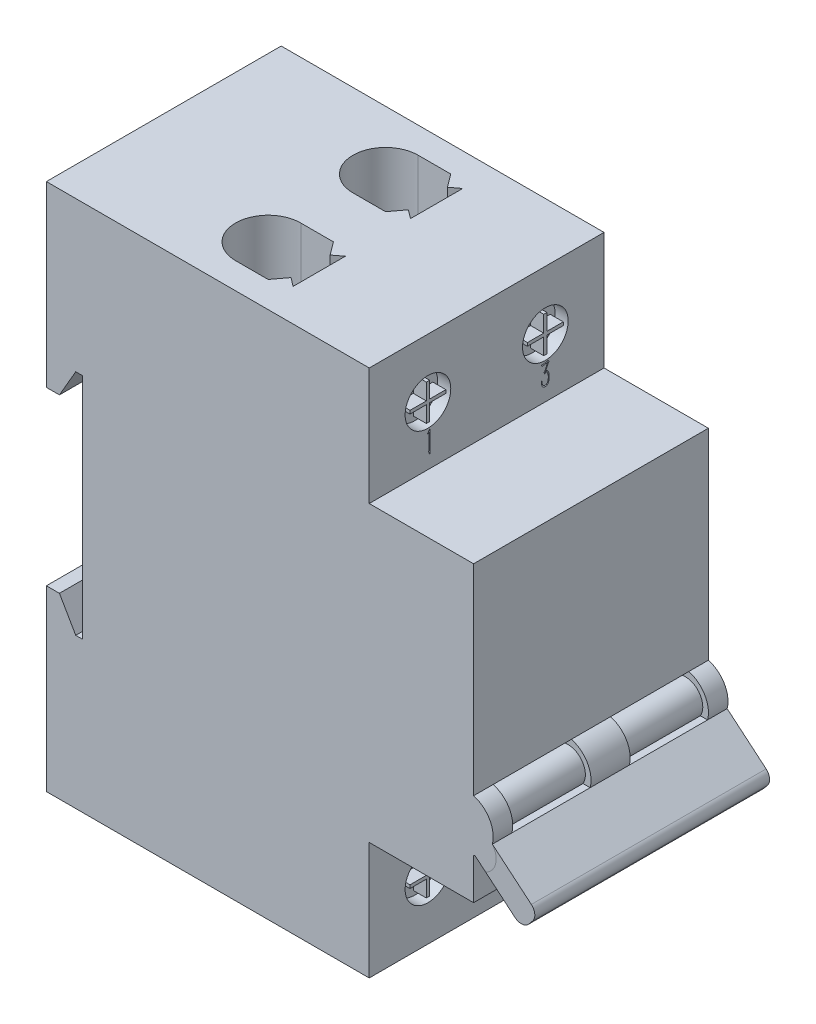
from build123d import *

# Parameters (mm, degrees)
EXTRUDE_1_DEPTH        = 18
SKETCH_2_R             = 3.5
CUT_EXTRUDE_1_DEPTH    = 2
CUT_EXTRUDE_5_DEPTH    = 15
SKETCH_12_R            = 4.114641301
EXTRUDE_4_DEPTH        = 18
EXTRUDE_5_DEPTH        = 18
FILLET_1_R             = 1.5
SKETCH_15_W            = 12
SKETCH_15_H            = 4.990244444
CUT_EXTRUDE_9_DEPTH    = 5
EXTRUDE_6_REACH        = 88.448
SKETCH_16_R            = 2.68605677
PATTERN_LINEAR_2_COUNT = 2
PATTERN_LINEAR_2_PITCH = 18
CUT_EXTRUDE_10_DEPTH   = 1


with BuildPart() as part:
    # 草图1 → 凸台-拉伸1 (new body)
    with BuildSketch(Plane.XY):
        Polygon((0, 13.169872981), (2, 13.169872981), (4.5, 17.5), (5.5, 17.5), (5.5, -17.5), (4.5, -17.5), (2, -13.169872981), (0, -13.169872981), (0, -40.5), (49.5, -40.5), (49.5, -22.5), (65.5, -22.5), (65.5, 22.5), (49.5, 22.5), (49.5, 40.5), (0, 40.5), align=None)
    extrude(amount=-EXTRUDE_1_DEPTH)

    # 草图2 → 切除-拉伸1 (cut)
    with BuildSketch(Plane(origin=(49.5, 0, 0), x_dir=(0, 0, -1), z_dir=(1, 0, 0))):
        with Locations((9, 31.5)):
            Circle(SKETCH_2_R)
        Polygon((8.75, 34.25), (9.25, 34.25), (9.25, 31.75), (11.75, 31.75), (11.75, 31.25), (9.25, 31.25), (9.25, 28.75), (8.75, 28.75), (8.75, 31.25), (6.25, 31.25), (6.25, 31.75), (8.75, 31.75), align=None, mode=Mode.SUBTRACT)
    cut_extrude_1 = extrude(amount=-CUT_EXTRUDE_1_DEPTH, mode=Mode.SUBTRACT)

    # 草图11 → 切除-拉伸5 (cut)
    with BuildSketch(Plane(origin=(0, 40.5, 0), x_dir=(1, 0, 0), z_dir=(0, 1, 0))):
        with BuildLine():
            Line((32.833333333, 5), (32.833333333, 13))
            Line((32.833333333, 13), (31.5, 12))
            Line((31.5, 12), (30, 14))
            Line((30, 14), (25, 14))
            ThreePointArc((25, 14), (21.464466094, 12.535533906), (20, 9))
            ThreePointArc((20, 9), (21.464466094, 5.464466094), (25, 4))
            Line((25, 4), (30, 4))
            Line((30, 4), (31.5, 6))
            Line((31.5, 6), (32.833333333, 5))
        make_face()
    cut_extrude_5 = extrude(amount=-CUT_EXTRUDE_5_DEPTH, mode=Mode.SUBTRACT)

    # 镜向1: 切除-拉伸1, 切除-拉伸5 across plane
    add(cut_extrude_1.mirror(Plane.ZX), mode=Mode.SUBTRACT)
    add(cut_extrude_5.mirror(Plane.ZX), mode=Mode.SUBTRACT)

    # 草图12 → 凸台-拉伸4 (add, through all)
    with BuildSketch(Plane.XY):
        with Locations((64.39025967, -12.26560275)):
            Circle(SKETCH_12_R)
    extrude(amount=-EXTRUDE_4_DEPTH)

    # 草图13 → 凸台-拉伸5 (add, through all)
    with BuildSketch(Plane.XY):
        Polygon((65.5, -10.881779635), (75.5, -19.272775947), (72.999147741, -22.253175611), (65.5, -15.960643508), align=None)
    extrude(amount=-EXTRUDE_5_DEPTH)

    # 圆角1
    fillet_1_edges = [part.edges().sort_by_distance(p)[0] for p in [
        (75.5, -19.272775947, -9),
        (72.999147741, -22.253175611, -9),
    ]]
    fillet(fillet_1_edges, radius=FILLET_1_R)

    # 草图15 → 切除-拉伸9 (cut, symmetric)
    with BuildSketch(Plane(origin=(65.5, 0, 0), x_dir=(0, 0, -1), z_dir=(1, 0, 0))):
        with Locations((9, -10.798560231)):
            Rectangle(SKETCH_15_W, SKETCH_15_H)
    extrude(amount=CUT_EXTRUDE_9_DEPTH, both=True, mode=Mode.SUBTRACT)

    # 草图16 → 凸台-拉伸6 (add, up to next)
    with BuildSketch(Plane.XY.offset(-15), mode=Mode.PRIVATE) as extrude_6_sk1:
        with Locations((64.953909061, -11.94282373)):
            Circle(SKETCH_16_R)
    extrude_6_tool1 = extrude(extrude_6_sk1.sketch, amount=EXTRUDE_6_REACH, mode=Mode.PRIVATE) - part.part
    add(extrude_6_tool1.solids().sort_by_distance((64.953909, -11.942824, -15))[0])


with BuildPart() as pattern_linear_2_1:
    # 阵列(线性)2: pattern copy
    add(part.part.moved(Location(Vector(0, 0, -1) * (1 * PATTERN_LINEAR_2_PITCH))))


with BuildPart() as part_1:
    add(part.part)

    # Combine 1: union 阵列(线性)2_1
    add(pattern_linear_2_1.part)

    # 草图19 → 切除-拉伸10 (cut)
    # profile 1 of 4: a face of its own
    with BuildSketch(Plane(origin=(49.5, 0, 0), x_dir=(0, 0, -1), z_dir=(1, 0, 0))):
        with BuildLine():
            Line((9.268616193, 27.777022397), (9.323804772, 27.777022397))
            Line((9.323804772, 27.777022397), (9.31858423, 25.103359495))
            add(Edge.make_bspline(
                [(9.31858423, 25.103359495), (9.317989513, 25.079247206), (9.316849208, 25.033014576), (9.316756663, 24.966867672), (9.314581251, 24.906977786), (9.31440798, 24.853259172), (9.312790378, 24.805782007), (9.310919778, 24.764536358), (9.310742036, 24.729444909), (9.307433278, 24.674522263), (9.303490456, 24.59900772), (9.293712461, 24.521229024), (9.285928441, 24.465808449), (9.278015344, 24.440580035), (9.267990261, 24.420618486), (9.257985248, 24.422946371), (9.253700361, 24.423943344)],
                knots=[0, 0, 0, 0, 1.45038606, 2.780953852, 3.977268029, 5.053718292, 6.010937745, 6.833690271, 7.536464333, 8.120251454, 10.142880859, 12.069479857, 12.873132744, 13.440417135, 13.76034519, 14, 14, 14, 14], degree=3))
            add(Edge.make_bspline(
                [(9.253700361, 24.423943344), (9.252709832, 24.424693106), (9.248470125, 24.427902274), (9.238359598, 24.434694901), (9.226346206, 24.452902941), (9.221087494, 24.469237998), (9.217902364, 24.479131922)],
                knots=[0, 0, 0, 0, 0.221265066, 0.947068446, 2.150880552, 4, 4, 4, 4], degree=3))
            Line((9.217902364, 24.479131922), (9.193291241, 24.544761583))
            Line((9.193291241, 24.544761583), (9.13735687, 24.725988943))
            add(Edge.make_bspline(
                [(9.13735687, 24.725988943), (9.130623579, 24.743040571), (9.118894532, 24.772743625), (9.107062513, 24.811822119), (9.098086344, 24.836775388), (9.09570055, 24.857001098), (9.107192928, 24.875972867), (9.11565667, 24.905183607), (9.128680107, 24.942469195), (9.140978693, 24.986476292), (9.151841244, 25.034025265), (9.161626509, 25.085400436), (9.167172099, 25.143283169), (9.169892428, 25.198549028), (9.171980118, 25.251758462), (9.172359418, 25.302984326), (9.173405582, 25.363637315), (9.173242151, 25.407393199), (9.173154868, 25.43076201)],
                knots=[0, 0, 0, 0, 1.220359697, 2.125803599, 2.712350858, 2.994193817, 3.439826662, 4.12562012, 5.031064022, 6.063176816, 7.167225426, 8.277459231, 9.542238136, 11.034069985, 11.961482632, 13.08703073, 14.444263491, 16, 16, 16, 16], degree=3))
            Line((9.173154868, 25.43076201), (9.177629617, 27.404126595))
            Line((9.177629617, 27.404126595), (8.915856764, 27.177405947))
            Line((8.915856764, 27.177405947), (8.895720391, 27.263171982))
            add(Edge.make_bspline(
                [(8.895720391, 27.263171982), (8.916998829, 27.285159101), (8.956886141, 27.326374863), (9.010193269, 27.385718152), (9.054036517, 27.437218727), (9.099702186, 27.497425312), (9.150830111, 27.572352034), (9.188586471, 27.633910013), (9.208207073, 27.665899448)],
                knots=[0, 0, 0, 0, 1.077185482, 2.019228619, 2.808185376, 3.45765616, 4.678836699, 6, 6, 6, 6], degree=3))
            Line((9.208207073, 27.665899448), (9.268616193, 27.777022397))
        make_face()
    # profile 2 of 4: a face of its own
    with BuildSketch(Plane(origin=(49.5, 0, 0), x_dir=(0, 0, -1), z_dir=(1, 0, 0))):
        with BuildLine():
            add(Edge.make_bspline(
                [(26.894587034, 26.553178374), (26.905758668, 26.576305419), (26.92727936, 26.620856647), (26.95866931, 26.685209589), (26.987953271, 26.744293665), (27.012999895, 26.799120123), (27.036354733, 26.848480227), (27.057155241, 26.892902394), (27.075128281, 26.932401147), (27.094050096, 26.976253222), (27.113674908, 27.02200111), (27.132673375, 27.066809999), (27.146489283, 27.098818021), (27.153632136, 27.115750937), (27.156359887, 27.122217369)],
                knots=[0, 0, 0, 0, 1.475873638, 2.843077615, 4.114458223, 5.26483622, 6.306479236, 7.252326145, 8.083448402, 8.799989154, 9.996708352, 10.943956596, 11.596712522, 12, 12, 12, 12], degree=3))
            Line((27.156359887, 27.122217369), (27.317450874, 27.55030175))
            add(Edge.make_bspline(
                [(27.317450874, 27.55030175), (27.282414717, 27.546873059), (27.20596755, 27.539391824), (27.108407493, 27.533451709), (27.027289802, 27.529125888), (26.971629196, 27.524461766), (26.922889389, 27.520102343), (26.892842398, 27.516785719), (26.87892541, 27.515249544)],
                knots=[0, 0, 0, 0, 1.440114021, 3.142257811, 3.998086789, 4.76330671, 5.427195687, 6, 6, 6, 6], degree=3))
            Line((26.87892541, 27.515249544), (26.728275506, 27.48989263))
            add(Edge.make_bspline(
                [(26.728275506, 27.48989263), (26.721544061, 27.488477454), (26.70317884, 27.484616469), (26.669215876, 27.474073313), (26.620302936, 27.461107664), (26.58307352, 27.450445131), (26.561963978, 27.444399342)],
                knots=[0, 0, 0, 0, 0.478461291, 1.305373098, 2.472113022, 4, 4, 4, 4], degree=3))
            Line((26.561963978, 27.444399342), (26.511995941, 27.424262968))
            Line((26.511995941, 27.424262968), (26.38595716, 27.61071087))
            add(Edge.make_bspline(
                [(26.38595716, 27.61071087), (26.380634962, 27.618010698), (26.371549402, 27.630472284), (26.364006769, 27.647807605), (26.358407972, 27.65985087), (26.363426008, 27.671978454), (26.383268796, 27.670159902), (26.398250403, 27.659523203), (26.417386103, 27.649289333), (26.439402155, 27.647850003), (26.466093406, 27.646283592), (26.485655754, 27.64932396), (26.496334317, 27.650983616)],
                knots=[0, 0, 0, 0, 1.323589942, 2.259509366, 2.829398404, 3.190947808, 3.965341466, 5.19662492, 6.050472624, 7.088782, 8.410843841, 10, 10, 10, 10], degree=3))
            Line((26.496334317, 27.650983616), (26.657425304, 27.656204158))
            Line((26.657425304, 27.656204158), (27.292093959, 27.73152911))
            Line((27.292093959, 27.73152911), (27.342061997, 27.777022397))
            Line((27.342061997, 27.777022397), (27.382334743, 27.817295144))
            add(Edge.make_bspline(
                [(27.382334743, 27.817295144), (27.383583719, 27.815808411), (27.388703828, 27.809713632), (27.399726504, 27.795210802), (27.419326367, 27.771910062), (27.434144734, 27.752492469), (27.442743863, 27.7412244)],
                knots=[0, 0, 0, 0, 0.23984028, 0.983211964, 2.249351781, 4, 4, 4, 4], degree=3))
            Line((27.442743863, 27.7412244), (27.53895098, 27.62040616))
            add(Edge.make_bspline(
                [(27.53895098, 27.62040616), (27.54541144, 27.612018118), (27.556147701, 27.598078521), (27.564112726, 27.575785092), (27.555951012, 27.56068078), (27.544549588, 27.547733644), (27.52606782, 27.532183142), (27.511424617, 27.521362113), (27.503152983, 27.515249544)],
                knots=[0, 0, 0, 0, 1.419029252, 2.358201718, 2.827787952, 3.596253847, 4.642174893, 6, 6, 6, 6], degree=3))
            Line((27.503152983, 27.515249544), (27.447964405, 27.469756256))
            add(Edge.make_bspline(
                [(27.447964405, 27.469756256), (27.43183587, 27.429222959), (27.401234241, 27.352316717), (27.357143356, 27.242865851), (27.316798395, 27.145548297), (27.281372724, 27.059514144), (27.248833746, 26.985741252), (27.221970898, 26.923143149), (27.197785591, 26.872921774), (27.182992591, 26.843523203), (27.176496261, 26.830612851)],
                knots=[0, 0, 0, 0, 1.507300768, 2.859891598, 4.076963614, 5.147345159, 6.074452096, 6.862861548, 7.500626815, 8, 8, 8, 8], degree=3))
            Line((27.176496261, 26.830612851), (27.025100565, 26.543483084))
            add(Edge.make_bspline(
                [(27.025100565, 26.543483084), (27.042996023, 26.54491193), (27.077268983, 26.547648422), (27.129573753, 26.552872254), (27.186562807, 26.54568692), (27.236547135, 26.525696313), (27.279075075, 26.501029434), (27.313152721, 26.476392071), (27.345708772, 26.444370394), (27.378905936, 26.406726573), (27.412180649, 26.361796719), (27.442768582, 26.307377441), (27.474610228, 26.245235491), (27.514431877, 26.150532156), (27.557460863, 26.023817162), (27.583604576, 25.86466242), (27.596521571, 25.705205737), (27.598417879, 25.599087053), (27.5993601, 25.546359708)],
                knots=[0, 0, 0, 0, 0.660541429, 1.265053373, 1.928435853, 2.750244091, 3.225390118, 3.735570922, 4.291687282, 4.900607759, 5.580848831, 6.342918567, 7.193367346, 8.147740655, 10.119512469, 12.097611575, 14.061014616, 16, 16, 16, 16], degree=3))
            add(Edge.make_bspline(
                [(27.5993601, 25.546359708), (27.597369738, 25.505079829), (27.593588689, 25.426661312), (27.584450789, 25.315849931), (27.570814377, 25.218634004), (27.550955275, 25.109031476), (27.515932295, 24.987942252), (27.472665848, 24.876226259), (27.431585008, 24.795741244), (27.396962993, 24.742372127), (27.359042011, 24.69462663), (27.318290969, 24.652844146), (27.275901478, 24.618507711), (27.234760539, 24.588977252), (27.193130085, 24.568106084), (27.139235736, 24.550670286), (27.073375552, 24.538651683), (27.020920749, 24.536243809), (26.995268901, 24.535066293)],
                knots=[0, 0, 0, 0, 1.512752116, 2.8737433, 4.067977017, 5.104892351, 6.948544146, 8.672095895, 9.482011449, 10.251829035, 10.996496654, 11.710742831, 12.38300564, 12.991319199, 13.561044299, 14.079002633, 15.060579187, 16, 16, 16, 16], degree=3))
            add(Edge.make_bspline(
                [(26.995268901, 24.535066293), (26.973388966, 24.534693339), (26.93129448, 24.53397582), (26.870237534, 24.538946321), (26.81462808, 24.55032289), (26.762475647, 24.565798969), (26.713633203, 24.590272598), (26.666979223, 24.625233083), (26.620013623, 24.668282899), (26.574983014, 24.721112889), (26.533770386, 24.781638563), (26.497735149, 24.848588226), (26.46779483, 24.921014069), (26.438030374, 25.024086001), (26.412802475, 25.155884677), (26.408308057, 25.262588435), (26.406093533, 25.315164311)],
                knots=[0, 0, 0, 0, 0.828828519, 1.594571005, 2.314948186, 2.97625877, 3.650192192, 4.371738268, 5.178272596, 6.059897072, 6.995131469, 7.947518938, 8.935744196, 9.957858231, 12.008325587, 14, 14, 14, 14], degree=3))
            Line((26.406093533, 25.315164311), (26.400872992, 25.511307503))
            Line((26.400872992, 25.511307503), (26.456061571, 25.511307503))
            add(Edge.make_bspline(
                [(26.456061571, 25.511307503), (26.460281768, 25.482221028), (26.468363821, 25.426517849), (26.480120095, 25.346152318), (26.492296408, 25.272893692), (26.50601877, 25.186199105), (26.528872927, 25.088850434), (26.567375212, 24.984077852), (26.619589704, 24.89555163), (26.680895946, 24.822599949), (26.752597249, 24.769647856), (26.829354682, 24.736246775), (26.90758436, 24.720476219), (26.959416586, 24.720672281), (26.984827818, 24.720768402)],
                knots=[0, 0, 0, 0, 0.994021113, 1.903638599, 2.746793397, 3.505624798, 4.871908371, 6.122639036, 7.264652637, 8.331625701, 9.323760524, 10.250011688, 11.142051883, 12, 12, 12, 12], degree=3))
            add(Edge.make_bspline(
                [(26.984827818, 24.720768402), (27.005270774, 24.722531252), (27.045310018, 24.725983941), (27.103371268, 24.739128694), (27.157066245, 24.761557691), (27.207260378, 24.790239493), (27.252440104, 24.827641551), (27.293102101, 24.871713388), (27.327537611, 24.924069674), (27.366130118, 25.004224122), (27.403636112, 25.114727617), (27.431856393, 25.255086396), (27.450219792, 25.398256076), (27.458846817, 25.540709206), (27.460022294, 25.681050273), (27.448482407, 25.772899132), (27.442743863, 25.818573644)],
                knots=[0, 0, 0, 0, 0.647840119, 1.268849254, 1.871153999, 2.479976942, 3.088343857, 3.716462885, 4.367721208, 5.059616847, 6.52246665, 8.039623249, 9.575767262, 11.078710543, 12.547304005, 14, 14, 14, 14], degree=3))
            add(Edge.make_bspline(
                [(27.442743863, 25.818573644), (27.434719682, 25.867804036), (27.418857721, 25.965121191), (27.382165945, 26.081930294), (27.346034778, 26.169154367), (27.313799504, 26.227674778), (27.277262229, 26.279947351), (27.235874793, 26.32378913), (27.193919543, 26.35976614), (27.15180766, 26.383772702), (27.110219955, 26.396125961), (27.083571503, 26.393410031), (27.070593853, 26.392087388)],
                knots=[0, 0, 0, 0, 2.019199264, 3.991492233, 4.943861116, 5.841091039, 6.693606335, 7.520378909, 8.278781735, 8.923571305, 9.475785111, 10, 10, 10, 10], degree=3))
            Line((27.070593853, 26.392087388), (26.990048359, 26.382392097))
            Line((26.990048359, 26.382392097), (26.954996154, 26.316762436))
            add(Edge.make_bspline(
                [(26.954996154, 26.316762436), (26.950317629, 26.308583345), (26.94216181, 26.294325183), (26.931016972, 26.275479105), (26.922115728, 26.264440522), (26.915359483, 26.254924454), (26.905592767, 26.258125672), (26.899310799, 26.269064642), (26.889268494, 26.285168339), (26.882736067, 26.298999064), (26.87892541, 26.307067145)],
                knots=[0, 0, 0, 0, 1.659028505, 2.892093886, 3.763458346, 4.288089223, 4.647361994, 5.327919393, 6.441255868, 8, 8, 8, 8], degree=3))
            Line((26.87892541, 26.307067145), (26.798379917, 26.46293759))
            add(Edge.make_bspline(
                [(26.798379917, 26.46293759), (26.792557932, 26.471896017), (26.782408552, 26.48751311), (26.786808583, 26.505315301), (26.788684626, 26.512905628)],
                knots=[0, 0, 0, 0, 1.147259222, 2, 2, 2, 2], degree=3))
            Line((26.788684626, 26.512905628), (26.828957373, 26.528567251))
            Line((26.828957373, 26.528567251), (26.894587034, 26.553178374))
        make_face()
    # profile 3 of 4: a face of its own
    with BuildSketch(Plane(origin=(49.5, 0, 0), x_dir=(0, 0, -1), z_dir=(1, 0, 0))):
        with BuildLine():
            Line((8.730154654, -24.847385713), (8.654083911, -24.847385713))
            add(Edge.make_bspline(
                [(8.654083911, -24.847385713), (8.652516507, -24.823276458), (8.649528375, -24.777314072), (8.646445032, -24.711674798), (8.64514292, -24.652738754), (8.643838503, -24.580888811), (8.645850242, -24.490276951), (8.65125193, -24.417292602), (8.654083911, -24.379028585)],
                knots=[0, 0, 0, 0, 0.927540379, 1.768282303, 2.522502339, 3.190652681, 4.527123766, 6, 6, 6, 6], degree=3))
            add(Edge.make_bspline(
                [(8.654083911, -24.379028585), (8.656043818, -24.350662308), (8.659834054, -24.295805178), (8.669837058, -24.216742672), (8.681413565, -24.143478296), (8.69646412, -24.074567742), (8.7167999, -24.007131882), (8.745750083, -23.939303027), (8.781856415, -23.868757962), (8.824515086, -23.797966017), (8.871321724, -23.731168134), (8.923860232, -23.676810886), (8.978846052, -23.635379689), (9.03734966, -23.610721813), (9.093521598, -23.595388131), (9.144745804, -23.583326557), (9.190777383, -23.574897147), (9.219860114, -23.573997547), (9.233563987, -23.573573652)],
                knots=[0, 0, 0, 0, 1.238521709, 2.395159043, 3.470603583, 4.46912877, 5.466066804, 6.534123646, 7.677244524, 8.916145015, 10.13365226, 11.221244199, 12.198275335, 13.109907183, 13.966820176, 14.733954848, 15.403435577, 16, 16, 16, 16], degree=3))
            add(Edge.make_bspline(
                [(9.233563987, -23.573573652), (9.251028183, -23.574861334), (9.285536892, -23.577405754), (9.336298249, -23.589194749), (9.3853233, -23.606192719), (9.448027995, -23.63647274), (9.521351042, -23.683947637), (9.583729421, -23.746290041), (9.626893488, -23.803356357), (9.65729834, -23.851924205), (9.684241838, -23.90615696), (9.718077941, -23.984958998), (9.75347521, -24.089530022), (9.779001912, -24.221603947), (9.795369003, -24.35875684), (9.802857469, -24.498968402), (9.804249869, -24.637798018), (9.796098136, -24.728340443), (9.792161899, -24.772060761)],
                knots=[0, 0, 0, 0, 0.570779476, 1.127842599, 1.694919432, 2.261066821, 3.397481896, 4.527710891, 5.118384485, 5.730727279, 6.394748858, 7.092559246, 8.529363642, 9.986910621, 11.474321506, 13.03467297, 14.568129345, 16, 16, 16, 16], degree=3))
            add(Edge.make_bspline(
                [(9.792161899, -24.772060761), (9.784182525, -24.817033009), (9.768104722, -24.907648497), (9.733475036, -25.016748296), (9.701178927, -25.099692259), (9.674177686, -25.155273163), (9.645327126, -25.204477751), (9.603609389, -25.262667052), (9.539900956, -25.328718412), (9.480864698, -25.373013219), (9.449843553, -25.396288334)],
                knots=[0, 0, 0, 0, 1.490916612, 3.004077927, 3.729534125, 4.397912905, 5.020560084, 5.590839424, 6.734084393, 8, 8, 8, 8], degree=3))
            Line((9.449843553, -25.396288334), (9.202986532, -25.552158779))
            add(Edge.make_bspline(
                [(9.202986532, -25.552158779), (9.171529528, -25.573514544), (9.111881044, -25.614009149), (9.032233852, -25.680155183), (8.965383351, -25.749851267), (8.914854257, -25.826914516), (8.875609345, -25.906240314), (8.840761113, -25.985891172), (8.814452469, -26.073684748), (8.795740738, -26.152376603), (8.782979957, -26.218465922), (8.776587827, -26.264558022), (8.771395086, -26.305294785), (8.770736473, -26.330751604), (8.770427401, -26.34269788)],
                knots=[0, 0, 0, 0, 1.453572249, 2.75625039, 3.953730064, 5.132566341, 6.263730064, 7.337486329, 8.453238547, 9.76321854, 10.430854957, 11.026567013, 11.543191201, 12, 12, 12, 12], degree=3))
            Line((8.770427401, -26.34269788), (8.759986319, -26.553756904))
            Line((8.759986319, -26.553756904), (9.660902577, -26.52392524))
            add(Edge.make_bspline(
                [(9.660902577, -26.52392524), (9.672462855, -26.523278875), (9.692767296, -26.522143602), (9.71228111, -26.500870216), (9.71662466, -26.474895395), (9.724332018, -26.442947113), (9.730061911, -26.397152102), (9.734482123, -26.362325748), (9.736973321, -26.34269788)],
                knots=[0, 0, 0, 0, 0.925905201, 1.626257371, 2.181371879, 3.087088273, 4.358305093, 6, 6, 6, 6], degree=3))
            Line((9.736973321, -26.34269788), (9.757109694, -25.904172416))
            Line((9.757109694, -25.904172416), (9.827214105, -25.904172416))
            Line((9.827214105, -25.904172416), (9.852571019, -26.568672736))
            add(Edge.make_bspline(
                [(9.852571019, -26.568672736), (9.853418715, -26.581591346), (9.854901335, -26.604186009), (9.855623054, -26.634075483), (9.855643482, -26.654888005), (9.855328713, -26.671692005), (9.849916523, -26.68638406), (9.84488751, -26.703431679), (9.825269802, -26.713062781), (9.797070739, -26.716144309), (9.754214435, -26.720508585), (9.720578586, -26.720229453), (9.701175324, -26.720068432)],
                knots=[0, 0, 0, 0, 1.385018147, 2.4223982, 3.193529914, 3.619812046, 4.200562765, 4.878496499, 5.402948042, 6.404258339, 7.925751149, 10, 10, 10, 10], degree=3))
            Line((9.701175324, -26.720068432), (8.699577199, -26.745425346))
            add(Edge.make_bspline(
                [(8.699577199, -26.745425346), (8.687401759, -26.745460965), (8.663403069, -26.745531172), (8.638810076, -26.721667198), (8.628486444, -26.692453054), (8.623319507, -26.658091359), (8.61985857, -26.612504766), (8.618196149, -26.534098628), (8.621750352, -26.422538741), (8.629756092, -26.330484316), (8.633947537, -26.28228876)],
                knots=[0, 0, 0, 0, 0.556373901, 1.096654043, 1.476064089, 2.012759395, 2.73145082, 3.635924119, 5.715166189, 8, 8, 8, 8], degree=3))
            add(Edge.make_bspline(
                [(8.633947537, -26.28228876), (8.637667097, -26.254157079), (8.644832261, -26.199965695), (8.659400716, -26.121959966), (8.674933052, -26.049553187), (8.691789735, -25.982789164), (8.710398684, -25.922019627), (8.7307103, -25.867314144), (8.751766421, -25.81779166), (8.783393806, -25.761768771), (8.82358975, -25.700701936), (8.86931043, -25.634857188), (8.91333054, -25.579003158), (8.970866969, -25.517554724), (9.048760279, -25.450483145), (9.114195614, -25.401371673), (9.147797953, -25.37615196)],
                knots=[0, 0, 0, 0, 1.103491021, 2.125706759, 3.085324024, 3.98349739, 4.803138144, 5.555704107, 6.252741852, 6.89323317, 8.054555834, 9.09539633, 10.010480884, 10.817709087, 12.365830683, 14, 14, 14, 14], degree=3))
            Line((9.147797953, -25.37615196), (9.354382227, -25.244892638))
            add(Edge.make_bspline(
                [(9.354382227, -25.244892638), (9.370921509, -25.233896319), (9.402660187, -25.212794517), (9.446498042, -25.179198736), (9.483871457, -25.144340724), (9.516078649, -25.106724377), (9.545234203, -25.063196929), (9.569178512, -25.008940647), (9.59449199, -24.945031971), (9.624006101, -24.845602012), (9.654437281, -24.714363208), (9.666102897, -24.552212497), (9.65987102, -24.387958902), (9.640818996, -24.278938888), (9.631070913, -24.22315814)],
                knots=[0, 0, 0, 0, 0.635613896, 1.219735276, 1.765761318, 2.268061313, 2.802129131, 3.435697723, 4.161225462, 5.001884758, 6.75303811, 8.46119913, 10.189351173, 12, 12, 12, 12], degree=3))
            add(Edge.make_bspline(
                [(9.631070913, -24.22315814), (9.623725567, -24.194721139), (9.609399703, -24.139259545), (9.582284963, -24.059364957), (9.547186593, -23.986598886), (9.509619076, -23.918624202), (9.462554079, -23.859122868), (9.399862794, -23.816389074), (9.325801546, -23.787822518), (9.27162761, -23.782792113), (9.243259278, -23.780157927)],
                knots=[0, 0, 0, 0, 1.101106684, 2.147523679, 3.156537618, 4.125318695, 5.058520457, 5.968677808, 6.93629249, 8, 8, 8, 8], degree=3))
            add(Edge.make_bspline(
                [(9.243259278, -23.780157927), (9.228326882, -23.78000505), (9.198543172, -23.779700127), (9.15418165, -23.786427429), (9.111033958, -23.800532746), (9.054355541, -23.826097853), (8.988862492, -23.873718727), (8.91992613, -23.945569602), (8.863064593, -24.033301084), (8.819285565, -24.13496587), (8.786366995, -24.250789776), (8.759643561, -24.380596909), (8.742096183, -24.52603338), (8.737193746, -24.627827981), (8.734629404, -24.681074185)],
                knots=[0, 0, 0, 0, 0.469335518, 0.936122588, 1.403629858, 1.893624907, 2.887406355, 3.927357629, 5.011993806, 6.157121359, 7.396943717, 8.794309501, 10.323183677, 12, 12, 12, 12], degree=3))
            Line((8.734629404, -24.681074185), (8.730154654, -24.847385713))
        make_face()
    # profile 4 of 4: a face of its own
    with BuildSketch(Plane(origin=(49.5, 0, 0), x_dir=(0, 0, -1), z_dir=(1, 0, 0))):
        with BuildLine():
            Line((27.186191551, -25.808711091), (26.476197944, -25.848983838))
            Line((26.476197944, -25.848983838), (26.426229906, -25.92430879))
            add(Edge.make_bspline(
                [(26.426229906, -25.92430879), (26.422969209, -25.932202289), (26.418041285, -25.944131812), (26.399821496, -25.956434612), (26.386153034, -25.938787294), (26.379694111, -25.927278587), (26.375516077, -25.91983404)],
                knots=[0, 0, 0, 0, 1.282902353, 1.938863145, 2.666728425, 4, 4, 4, 4], degree=3))
            Line((26.375516077, -25.91983404), (26.280054752, -25.728165598))
            add(Edge.make_bspline(
                [(26.280054752, -25.728165598), (26.275970963, -25.716847246), (26.269236836, -25.698183401), (26.264334142, -25.673131982), (26.265728107, -25.655463636), (26.268963559, -25.646337108), (26.270359461, -25.642399563)],
                knots=[0, 0, 0, 0, 1.63130738, 2.690008936, 3.434818089, 4, 4, 4, 4], degree=3))
            Line((26.270359461, -25.642399563), (26.310632208, -25.632704272))
            Line((26.310632208, -25.632704272), (26.365820786, -25.602126817))
            Line((26.365820786, -25.602126817), (27.216769007, -23.548216738))
            Line((27.216769007, -23.548216738), (27.327146165, -23.548216738))
            Line((27.327146165, -23.548216738), (27.327146165, -25.62226319))
            add(Edge.make_bspline(
                [(27.327146165, -25.62226319), (27.337517711, -25.622341822), (27.355153283, -25.622475527), (27.371235704, -25.615458278), (27.377859994, -25.612567899)],
                knots=[0, 0, 0, 0, 1.176207474, 2, 2, 2, 2], degree=3))
            Line((27.377859994, -25.612567899), (27.453184946, -25.581990443))
            add(Edge.make_bspline(
                [(27.453184946, -25.581990443), (27.462922591, -25.578356102), (27.480279634, -25.571878005), (27.502629071, -25.562149087), (27.518450332, -25.554658262), (27.525822287, -25.549000794), (27.528509898, -25.546938238)],
                knots=[0, 0, 0, 0, 1.495147538, 2.665053038, 3.513315187, 4, 4, 4, 4], degree=3))
            Line((27.528509898, -25.546938238), (27.563562103, -25.517106574))
            Line((27.563562103, -25.517106574), (27.704516717, -25.662535937))
            add(Edge.make_bspline(
                [(27.704516717, -25.662535937), (27.711697463, -25.671177462), (27.723452054, -25.685323286), (27.728582435, -25.70926226), (27.723689862, -25.725451473), (27.714543829, -25.737110002), (27.698601358, -25.741996953), (27.686866477, -25.742677653), (27.679905594, -25.74308143)],
                knots=[0, 0, 0, 0, 1.690587597, 2.767423091, 3.557953073, 4.202677464, 4.933866242, 6, 6, 6, 6], degree=3))
            Line((27.679905594, -25.74308143), (27.327146165, -25.783354176))
            Line((27.327146165, -25.783354176), (27.327146165, -26.685016226))
            add(Edge.make_bspline(
                [(27.327146165, -26.685016226), (27.327128212, -26.687751147), (27.327067793, -26.696955205), (27.328226229, -26.716330922), (27.328695969, -26.747160979), (27.329300443, -26.7854712), (27.330335667, -26.823912608), (27.330001199, -26.855048118), (27.327983039, -26.874682486), (27.323236362, -26.887300824), (27.313944894, -26.889560225), (27.309175758, -26.887373218), (27.307009791, -26.88637996)],
                knots=[0, 0, 0, 0, 0.375701713, 1.264380521, 2.665139726, 4.612257271, 6.525225464, 7.960129458, 8.858599367, 9.286556546, 9.675980055, 10, 10, 10, 10], degree=3))
            add(Edge.make_bspline(
                [(27.307009791, -26.88637996), (27.302798935, -26.883877082), (27.290105158, -26.876332067), (27.278979998, -26.851983484), (27.265612394, -26.826711093), (27.259603022, -26.808412858), (27.257041754, -26.800613925)],
                knots=[0, 0, 0, 0, 0.572299195, 1.725216547, 3.030459198, 4, 4, 4, 4], degree=3))
            Line((27.257041754, -26.800613925), (27.211548466, -26.709627349))
            Line((27.211548466, -26.709627349), (27.186191551, -26.639522938))
            add(Edge.make_bspline(
                [(27.186191551, -26.639522938), (27.182335483, -26.631121959), (27.175357852, -26.615920221), (27.167714287, -26.594965646), (27.160889762, -26.579495575), (27.157090728, -26.561090907), (27.161547109, -26.532339541), (27.171368715, -26.492075887), (27.183163945, -26.449032995), (27.188705787, -26.409701413), (27.190980879, -26.375794404), (27.191266296, -26.353888053), (27.191412093, -26.34269788)],
                knots=[0, 0, 0, 0, 0.908031708, 1.643101311, 2.192199313, 2.565975908, 3.473020803, 5.002279505, 6.661670863, 7.846934984, 8.900174221, 10, 10, 10, 10], degree=3))
            Line((27.191412093, -26.34269788), (27.186191551, -25.808711091))
        make_face()
        Polygon((27.191412093, -25.642399563), (27.191412093, -23.971080578), (26.481418485, -25.67819756), align=None, mode=Mode.SUBTRACT)
    extrude(amount=-CUT_EXTRUDE_10_DEPTH, mode=Mode.SUBTRACT)


solid = part_1.part
